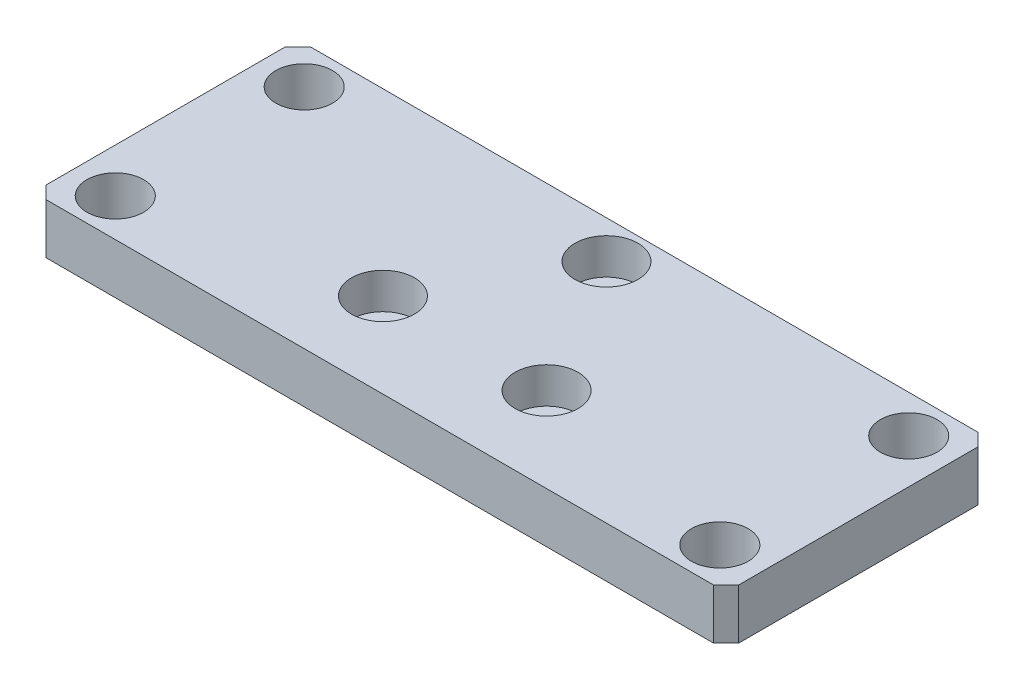
from build123d import *

# Parameters (mm, degrees)
SKETCH_1_W                   = 110
SKETCH_1_H                   = 42
EXTRUDE_1_DEPTH              = 4
HOLE_WIZARD_M6_1_D           = 5.5
HOLE_WIZARD_M6_1_CBORE_D     = 10
HOLE_WIZARD_M6_1_CBORE_DEPTH = 5.7
HOLE_WIZARD_9_0_9_1_D        = 9
CHAMFER_1_SIZE               = 2
MIRROR_2_COPY_1_D            = 9


with BuildPart() as part:
    # 草图1 → 凸台-拉伸1 (new, symmetric)
    with BuildSketch(Plane(origin=(0, 0, 0), x_dir=(1, 0, 0), z_dir=(0, 1, 0))):
        Rectangle(SKETCH_1_W, SKETCH_1_H)
    extrude(amount=EXTRUDE_1_DEPTH, both=True)

    # M6 六角凹头螺钉的柱形沉头孔1 (through all)
    with Locations(Plane(origin=(0, 4, 0), x_dir=(1, 0, 0), z_dir=(0, 1, 0))):
        with Locations((0, 15), (-12.990381057, -7.5), (12.990381057, -7.5)):
            CounterBoreHole(HOLE_WIZARD_M6_1_D / 2, HOLE_WIZARD_M6_1_CBORE_D / 2, HOLE_WIZARD_M6_1_CBORE_DEPTH)

    # Ø9.0 (9) 直径孔1 (through all)
    with Locations(Plane(origin=(0, -4, 0), x_dir=(-1, 0, 0), z_dir=(0, -1, 0))):
        with Locations((-48, -15)):
            hole_wizard_9_0_9_1 = Hole(HOLE_WIZARD_9_0_9_1_D / 2)

    # 倒角1
    chamfer_1_edges = [part.edges().sort_by_distance(p)[0] for p in [
        (55, 0, 21),
        (-55, 0, 21),
        (-55, 0, -21),
        (55, 0, -21),
    ]]
    chamfer(chamfer_1_edges, length=CHAMFER_1_SIZE)

    # 镜向1: Ø9.0 (9) 直径孔1 across plane
    add(hole_wizard_9_0_9_1.mirror(Plane.XY), mode=Mode.SUBTRACT)

    # 镜向2: Ø9.0 (9) 直径孔1 across plane
    add(hole_wizard_9_0_9_1.mirror(Plane(origin=(0, 0, 0), x_dir=(0, 0, 1), z_dir=(1, 0, 0))), mode=Mode.SUBTRACT)

    # 镜向2 copy 1 (through all)
    with Locations(Plane.XZ.offset(4)):
        with Locations((-48, -15)):
            Hole(MIRROR_2_COPY_1_D / 2)


solid = part.part
